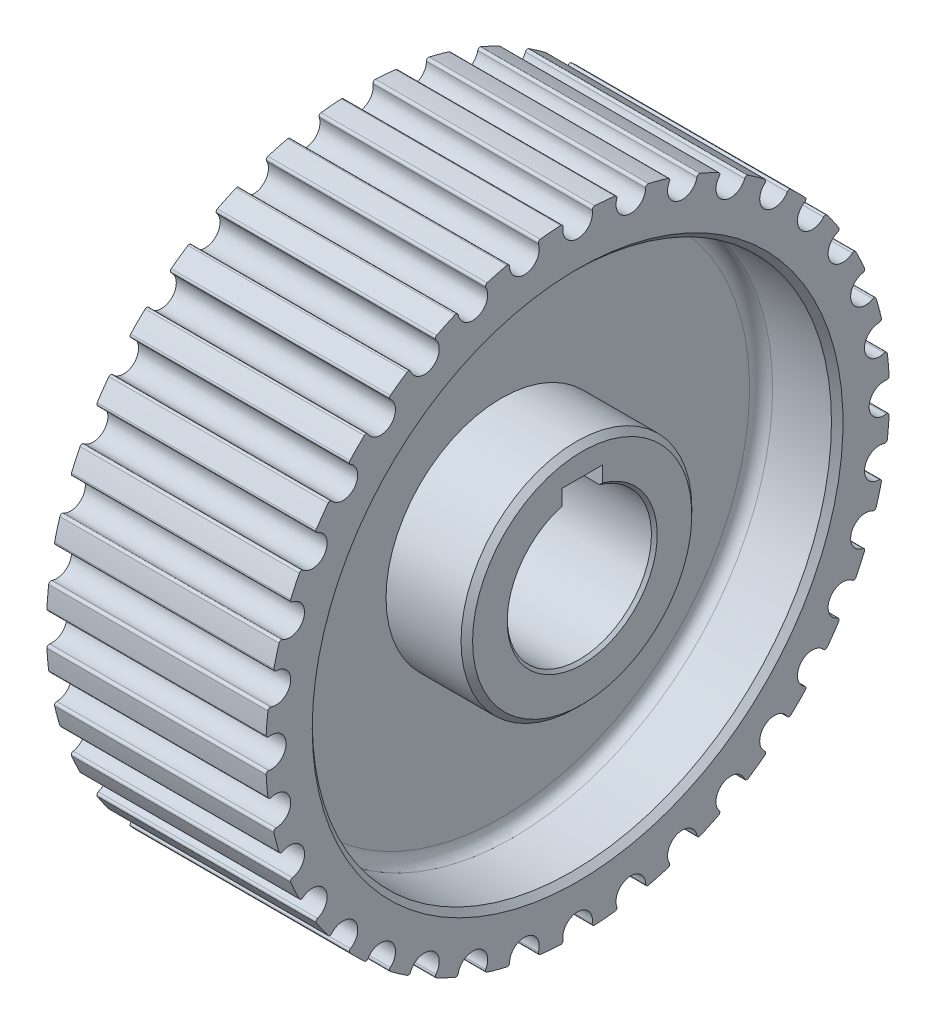
SolidWorks part; units mm, degrees
ref_plane "前视基准面" through (0, 0, 0) normal (0, 0, 1) x (1, 0, 0)
ref_plane "上视基准面" through (0, 0, 0) normal (0, 1, 0) x (1, 0, 0)
ref_plane "右视基准面" through (0, 0, 0) normal (1, 0, 0) x (0, 0, -1)
sketch "草图1" plane through (0, 0, 0) normal (0, 0, 1) x (1, 0, 0)
  line L0 (-38.4722, 0) -> (35.1779, 0) construction
  line L1 (-20.3293, 12.5) -> (17.6707, 12.5)
  line L2 (17.6707, 12.5) -> (17.6707, 20)
  line L3 (17.6707, 20) -> (3.6707, 20)
  line L4 (3.6707, 20) -> (3.6707, 45)
  line L5 (16.8769, 45) -> (3.6707, 45)
  line L6 (16.8769, 45) -> (16.8769, 54.07)
  line L7 (16.8769, 54.07) -> (-21.1231, 54.07)
  line L8 (-21.1231, 54.07) -> (-21.1231, 45)
  line L9 (-21.1231, 45) -> (-6.3293, 45)
  line L10 (-6.3293, 45) -> (-6.3293, 20)
  line L11 (-6.3293, 20) -> (-20.3293, 20)
  line L12 (-20.3293, 20) -> (-20.3293, 12.5)
  dimension "D1" = 38
  dimension "D2" = 7.5
  dimension "D3" = 14
  dimension "D4" = 14
  dimension "D5" = 7.5
  dimension "D6" = 25
  dimension "D7" = 9.07
  dimension "D8" = 12.5
revolve "旋转1" add sketch "草图1" angle 360 about L0
chamfer "倒角1" distance 1 angle 45 2 edges at (-21.1231, 0, 45) (16.8769, 0, 45)
fillet "圆角1" radius 2 2 edges at (-6.3293, 0, 45) (3.6707, 0, 45)
chamfer "倒角2" distance 1 angle 45 2 edges at (17.6707, 0, 20) (-20.3293, 0, 20)
chamfer "倒角3" distance 0.5 angle 45 2 edges at (-20.3293, 0, 12.5) (17.6707, 0, 12.5)
sketch "草图2" plane through (17.6707, 0, 0) normal (1, 0, 0) x (0, 0, -1)
  line L0 (0, -3.5835) -> (0, 27.7901) construction
  line L2 (-3.5, 12) -> (-3.5, 15.2)
  line L3 (-3.5, 15.2) -> (3.5, 15.2)
  line L4 (3.5, 12) -> (3.5, 15.2)
  arc A0 (3.5, 12) -> (-3.5, 12) centre (0, 0) ccw
  dimension "D1" = 25
  dimension "D2" = 3.2
  dimension "D3" = 7
  dimension "D4" = 3.5
extrude "切除-拉伸1" cut sketch "草图2" against normal through all
sketch "草图5" plane through (-21.1231, 0, 0) normal (-1, 0, 0) x (0, 0, 1)
  line L0 (0, 0) -> (0, 63.0632) construction
  arc A0 (-2.5348, 53.524) -> (2.5348, 53.524) centre (0, 53.1) ccw
  circle A1 centre (0, 0) radius 54.07 construction
  arc A2 (2.9511, 53.9894) -> (-2.9511, 53.9894) centre (0, 0) ccw
  arc A3 (-2.5348, 53.524) -> (-2.9511, 53.9894) centre (-2.9293, 53.59) ccw
  arc A4 (2.5348, 53.524) -> (2.9511, 53.9894) centre (2.9293, 53.59) cw
  point P8 (0, 50.53)
  point P9 (0, 54.07)
  point P12 (-2.5348, 53.524)
  dimension "D1" = 5.14
  dimension "D3" = 0.8
  dimension "D2" = 3.54
extrude "切除-拉伸2" cut sketch "草图5" against normal through all and the other way through all
pattern_circular "阵列(圆周)2" count 36 over 360 about axis through (0, 0, 0) along (1, 0, 0) of "切除-拉伸2"
sketch "草图6" plane through (-21.1231, 0, 0) normal (-1, 0, 0) x (0, 0, 1)
  arc A144 (-12.2815, 52.6567) -> (-15.6923, 51.7428) centre (0, 0) ccw
  arc A145 (-15.6923, 51.7428) -> (-15.9244, 51.1631) centre (-15.5762, 51.36) ccw
  arc A146 (-20.6882, 49.4292) -> (-15.9244, 51.1631) centre (-18.1613, 49.8977) ccw
  arc A147 (-20.6882, 49.4292) -> (-21.2386, 49.7241) centre (-21.0815, 49.3562) ccw
  arc A148 (-21.2386, 49.7241) -> (-24.4389, 48.2318) centre (0, 0) ccw
  arc A149 (-24.4389, 48.2318) -> (-24.5668, 47.6205) centre (-24.2582, 47.875) ccw
  arc A150 (-28.9572, 45.0858) -> (-24.5668, 47.6205) centre (-26.55, 45.9859) ccw
  arc A151 (-28.9572, 45.0858) -> (-29.5505, 45.2806) centre (-29.3318, 44.9457) ccw
  arc A152 (-29.5505, 45.2806) -> (-32.443, 43.2552) centre (0, 0) ccw
  arc A153 (-32.443, 43.2552) -> (-32.4628, 42.6311) centre (-32.203, 42.9352) ccw
  arc A154 (-36.3463, 39.3724) -> (-32.4628, 42.6311) centre (-34.132, 40.677) ccw
  arc A155 (-36.3463, 39.3724) -> (-36.9644, 39.4613) centre (-36.691, 39.1694) ccw
  arc A156 (-36.9644, 39.4613) -> (-39.4613, 36.9644) centre (0, 0) ccw
  arc A157 (-39.4613, 36.9644) -> (-39.3724, 36.3463) centre (-39.1694, 36.691) ccw
  arc A158 (-42.6311, 32.4628) -> (-39.3724, 36.3463) centre (-40.677, 34.132) ccw
  arc A159 (-42.6311, 32.4628) -> (-43.2552, 32.443) centre (-42.9352, 32.203) ccw
  arc A160 (-43.2552, 32.443) -> (-45.2806, 29.5505) centre (0, 0) ccw
  arc A161 (-45.2806, 29.5505) -> (-45.0858, 28.9572) centre (-44.9457, 29.3318) ccw
  arc A162 (-47.6205, 24.5668) -> (-45.0858, 28.9572) centre (-45.9859, 26.55) ccw
  arc A163 (-47.6205, 24.5668) -> (-48.2318, 24.4389) centre (-47.875, 24.2582) ccw
  arc A164 (-48.2318, 24.4389) -> (-49.7241, 21.2386) centre (0, 0) ccw
  arc A165 (-49.7241, 21.2386) -> (-49.4292, 20.6882) centre (-49.3562, 21.0815) ccw
  arc A166 (-51.1631, 15.9244) -> (-49.4292, 20.6882) centre (-49.8977, 18.1613) ccw
  arc A167 (-51.1631, 15.9244) -> (-51.7428, 15.6923) centre (-51.36, 15.5762) ccw
  arc A168 (-51.7428, 15.6923) -> (-52.6567, 12.2815) centre (0, 0) ccw
  arc A169 (-52.6567, 12.2815) -> (-52.2707, 11.7906) centre (-52.2672, 12.1906) ccw
  arc A170 (-53.151, 6.7981) -> (-52.2707, 11.7906) centre (-52.2933, 9.2207) ccw
  arc A171 (-53.151, 6.7981) -> (-53.6816, 6.4689) centre (-53.2845, 6.421) ccw
  arc A172 (-53.6816, 6.4689) -> (-53.9894, 2.9511) centre (0, 0) ccw
  arc A173 (-53.9894, 2.9511) -> (-53.524, 2.5348) centre (-53.59, 2.9293) ccw
  arc A174 (-53.524, -2.5348) -> (-53.524, 2.5348) centre (-53.1, 0) ccw
  arc A175 (-53.524, -2.5348) -> (-53.9894, -2.9511) centre (-53.59, -2.9293) ccw
  arc A176 (-53.9894, -2.9511) -> (-53.6816, -6.4689) centre (0, 0) ccw
  arc A177 (-53.6816, -6.4689) -> (-53.151, -6.7981) centre (-53.2845, -6.421) ccw
  arc A178 (-52.2707, -11.7906) -> (-53.151, -6.7981) centre (-52.2933, -9.2207) ccw
  arc A179 (-52.2707, -11.7906) -> (-52.6567, -12.2815) centre (-52.2672, -12.1906) ccw
  arc A180 (-52.6567, -12.2815) -> (-51.7428, -15.6923) centre (0, 0) ccw
  arc A181 (-51.7428, -15.6923) -> (-51.1631, -15.9244) centre (-51.36, -15.5762) ccw
  arc A182 (-49.4292, -20.6882) -> (-51.1631, -15.9244) centre (-49.8977, -18.1613) ccw
  arc A183 (-49.4292, -20.6882) -> (-49.7241, -21.2386) centre (-49.3562, -21.0815) ccw
  arc A184 (-49.7241, -21.2386) -> (-48.2318, -24.4389) centre (0, 0) ccw
  arc A185 (-48.2318, -24.4389) -> (-47.6205, -24.5668) centre (-47.875, -24.2582) ccw
  arc A186 (-45.0858, -28.9572) -> (-47.6205, -24.5668) centre (-45.9859, -26.55) ccw
  arc A187 (-45.0858, -28.9572) -> (-45.2806, -29.5505) centre (-44.9457, -29.3318) ccw
  arc A188 (-45.2806, -29.5505) -> (-43.2552, -32.443) centre (0, 0) ccw
  arc A189 (-43.2552, -32.443) -> (-42.6311, -32.4628) centre (-42.9352, -32.203) ccw
  arc A190 (-39.3724, -36.3463) -> (-42.6311, -32.4628) centre (-40.677, -34.132) ccw
  arc A191 (-39.3724, -36.3463) -> (-39.4613, -36.9644) centre (-39.1694, -36.691) ccw
  arc A192 (-39.4613, -36.9644) -> (-36.9644, -39.4613) centre (0, 0) ccw
  arc A193 (-36.9644, -39.4613) -> (-36.3463, -39.3724) centre (-36.691, -39.1694) ccw
  arc A194 (-32.4628, -42.6311) -> (-36.3463, -39.3724) centre (-34.132, -40.677) ccw
  arc A195 (-32.4628, -42.6311) -> (-32.443, -43.2552) centre (-32.203, -42.9352) ccw
  arc A196 (-32.443, -43.2552) -> (-29.5505, -45.2806) centre (0, 0) ccw
  arc A197 (-29.5505, -45.2806) -> (-28.9572, -45.0858) centre (-29.3318, -44.9457) ccw
  arc A198 (-24.5668, -47.6205) -> (-28.9572, -45.0858) centre (-26.55, -45.9859) ccw
  arc A199 (-24.5668, -47.6205) -> (-24.4389, -48.2318) centre (-24.2582, -47.875) ccw
  arc A200 (-24.4389, -48.2318) -> (-21.2386, -49.7241) centre (0, 0) ccw
  arc A201 (-21.2386, -49.7241) -> (-20.6882, -49.4292) centre (-21.0815, -49.3562) ccw
  arc A202 (-15.9244, -51.1631) -> (-20.6882, -49.4292) centre (-18.1613, -49.8977) ccw
  arc A203 (-15.9244, -51.1631) -> (-15.6923, -51.7428) centre (-15.5762, -51.36) ccw
  arc A204 (-15.6923, -51.7428) -> (-12.2815, -52.6567) centre (0, 0) ccw
  arc A205 (-12.2815, -52.6567) -> (-11.7906, -52.2707) centre (-12.1906, -52.2672) ccw
  arc A206 (-6.7981, -53.151) -> (-11.7906, -52.2707) centre (-9.2207, -52.2933) ccw
  arc A207 (-6.7981, -53.151) -> (-6.4689, -53.6816) centre (-6.421, -53.2845) ccw
  arc A208 (-6.4689, -53.6816) -> (-2.9511, -53.9894) centre (0, 0) ccw
  arc A209 (-2.9511, -53.9894) -> (-2.5348, -53.524) centre (-2.9293, -53.59) ccw
  arc A210 (2.5348, -53.524) -> (-2.5348, -53.524) centre (0, -53.1) ccw
  arc A211 (2.5348, -53.524) -> (2.9511, -53.9894) centre (2.9293, -53.59) ccw
  arc A212 (2.9511, -53.9894) -> (6.4689, -53.6816) centre (0, 0) ccw
  arc A213 (6.4689, -53.6816) -> (6.7981, -53.151) centre (6.421, -53.2845) ccw
  arc A214 (11.7906, -52.2707) -> (6.7981, -53.151) centre (9.2207, -52.2933) ccw
  arc A215 (11.7906, -52.2707) -> (12.2815, -52.6567) centre (12.1906, -52.2672) ccw
  arc A216 (12.2815, -52.6567) -> (15.6923, -51.7428) centre (0, 0) ccw
  arc A217 (15.6923, -51.7428) -> (15.9244, -51.1631) centre (15.5762, -51.36) ccw
  arc A218 (20.6882, -49.4292) -> (15.9244, -51.1631) centre (18.1613, -49.8977) ccw
  arc A219 (20.6882, -49.4292) -> (21.2386, -49.7241) centre (21.0815, -49.3562) ccw
  arc A220 (21.2386, -49.7241) -> (24.4389, -48.2318) centre (0, 0) ccw
  arc A221 (24.4389, -48.2318) -> (24.5668, -47.6205) centre (24.2582, -47.875) ccw
  arc A222 (28.9572, -45.0858) -> (24.5668, -47.6205) centre (26.55, -45.9859) ccw
  arc A223 (28.9572, -45.0858) -> (29.5505, -45.2806) centre (29.3318, -44.9457) ccw
  arc A224 (29.5505, -45.2806) -> (32.443, -43.2552) centre (0, 0) ccw
  arc A225 (32.443, -43.2552) -> (32.4628, -42.6311) centre (32.203, -42.9352) ccw
  arc A226 (36.3463, -39.3724) -> (32.4628, -42.6311) centre (34.132, -40.677) ccw
  arc A227 (36.3463, -39.3724) -> (36.9644, -39.4613) centre (36.691, -39.1694) ccw
  arc A228 (36.9644, -39.4613) -> (39.4613, -36.9644) centre (0, 0) ccw
  arc A229 (39.4613, -36.9644) -> (39.3724, -36.3463) centre (39.1694, -36.691) ccw
  arc A230 (42.6311, -32.4628) -> (39.3724, -36.3463) centre (40.677, -34.132) ccw
  arc A231 (42.6311, -32.4628) -> (43.2552, -32.443) centre (42.9352, -32.203) ccw
  arc A232 (43.2552, -32.443) -> (45.2806, -29.5505) centre (0, 0) ccw
  arc A233 (45.2806, -29.5505) -> (45.0858, -28.9572) centre (44.9457, -29.3318) ccw
  arc A234 (47.6205, -24.5668) -> (45.0858, -28.9572) centre (45.9859, -26.55) ccw
  arc A235 (47.6205, -24.5668) -> (48.2318, -24.4389) centre (47.875, -24.2582) ccw
  arc A236 (48.2318, -24.4389) -> (49.7241, -21.2386) centre (0, 0) ccw
  arc A237 (49.7241, -21.2386) -> (49.4292, -20.6882) centre (49.3562, -21.0815) ccw
  arc A238 (51.1631, -15.9244) -> (49.4292, -20.6882) centre (49.8977, -18.1613) ccw
  arc A239 (51.1631, -15.9244) -> (51.7428, -15.6923) centre (51.36, -15.5762) ccw
  arc A240 (51.7428, -15.6923) -> (52.6567, -12.2815) centre (0, 0) ccw
  arc A241 (52.6567, -12.2815) -> (52.2707, -11.7906) centre (52.2672, -12.1906) ccw
  arc A242 (53.151, -6.7981) -> (52.2707, -11.7906) centre (52.2933, -9.2207) ccw
  arc A243 (53.151, -6.7981) -> (53.6816, -6.4689) centre (53.2845, -6.421) ccw
  arc A244 (53.6816, -6.4689) -> (53.9894, -2.9511) centre (0, 0) ccw
  arc A245 (53.9894, -2.9511) -> (53.524, -2.5348) centre (53.59, -2.9293) ccw
  arc A246 (53.524, 2.5348) -> (53.524, -2.5348) centre (53.1, 0) ccw
  arc A247 (53.524, 2.5348) -> (53.9894, 2.9511) centre (53.59, 2.9293) ccw
  arc A248 (53.9894, 2.9511) -> (53.6816, 6.4689) centre (0, 0) ccw
  arc A249 (53.6816, 6.4689) -> (53.151, 6.7981) centre (53.2845, 6.421) ccw
  arc A250 (52.2707, 11.7906) -> (53.151, 6.7981) centre (52.2933, 9.2207) ccw
  arc A251 (52.2707, 11.7906) -> (52.6567, 12.2815) centre (52.2672, 12.1906) ccw
  arc A252 (52.6567, 12.2815) -> (51.7428, 15.6923) centre (0, 0) ccw
  arc A253 (51.7428, 15.6923) -> (51.1631, 15.9244) centre (51.36, 15.5762) ccw
  arc A254 (49.4292, 20.6882) -> (51.1631, 15.9244) centre (49.8977, 18.1613) ccw
  arc A255 (49.4292, 20.6882) -> (49.7241, 21.2386) centre (49.3562, 21.0815) ccw
  arc A256 (49.7241, 21.2386) -> (48.2318, 24.4389) centre (0, 0) ccw
  arc A257 (48.2318, 24.4389) -> (47.6205, 24.5668) centre (47.875, 24.2582) ccw
  arc A258 (45.0858, 28.9572) -> (47.6205, 24.5668) centre (45.9859, 26.55) ccw
  arc A259 (45.0858, 28.9572) -> (45.2806, 29.5505) centre (44.9457, 29.3318) ccw
  arc A260 (45.2806, 29.5505) -> (43.2552, 32.443) centre (0, 0) ccw
  arc A261 (43.2552, 32.443) -> (42.6311, 32.4628) centre (42.9352, 32.203) ccw
  arc A262 (39.3724, 36.3463) -> (42.6311, 32.4628) centre (40.677, 34.132) ccw
  arc A263 (39.3724, 36.3463) -> (39.4613, 36.9644) centre (39.1694, 36.691) ccw
  arc A264 (39.4613, 36.9644) -> (36.9644, 39.4613) centre (0, 0) ccw
  arc A265 (36.9644, 39.4613) -> (36.3463, 39.3724) centre (36.691, 39.1694) ccw
  arc A266 (32.4628, 42.6311) -> (36.3463, 39.3724) centre (34.132, 40.677) ccw
  arc A267 (32.4628, 42.6311) -> (32.443, 43.2552) centre (32.203, 42.9352) ccw
  arc A268 (32.443, 43.2552) -> (29.5505, 45.2806) centre (0, 0) ccw
  arc A269 (29.5505, 45.2806) -> (28.9572, 45.0858) centre (29.3318, 44.9457) ccw
  arc A270 (24.5668, 47.6205) -> (28.9572, 45.0858) centre (26.55, 45.9859) ccw
  arc A271 (24.5668, 47.6205) -> (24.4389, 48.2318) centre (24.2582, 47.875) ccw
  arc A272 (24.4389, 48.2318) -> (21.2386, 49.7241) centre (0, 0) ccw
  arc A273 (21.2386, 49.7241) -> (20.6882, 49.4292) centre (21.0815, 49.3562) ccw
  arc A274 (15.9244, 51.1631) -> (20.6882, 49.4292) centre (18.1613, 49.8977) ccw
  arc A275 (15.9244, 51.1631) -> (15.6923, 51.7428) centre (15.5762, 51.36) ccw
  arc A276 (15.6923, 51.7428) -> (12.2815, 52.6567) centre (0, 0) ccw
  arc A277 (12.2815, 52.6567) -> (11.7906, 52.2707) centre (12.1906, 52.2672) ccw
  arc A278 (6.7981, 53.151) -> (11.7906, 52.2707) centre (9.2207, 52.2933) ccw
  arc A279 (6.7981, 53.151) -> (6.4689, 53.6816) centre (6.421, 53.2845) ccw
  arc A280 (6.4689, 53.6816) -> (2.9511, 53.9894) centre (0, 0) ccw
  arc A281 (2.9511, 53.9894) -> (2.5348, 53.524) centre (2.9293, 53.59) ccw
  arc A282 (-2.5348, 53.524) -> (2.5348, 53.524) centre (0, 53.1) ccw
  arc A283 (-2.5348, 53.524) -> (-2.9511, 53.9894) centre (-2.9293, 53.59) ccw
  arc A284 (-2.9511, 53.9894) -> (-6.4689, 53.6816) centre (0, 0) ccw
  arc A285 (-6.4689, 53.6816) -> (-6.7981, 53.151) centre (-6.421, 53.2845) ccw
  arc A286 (-11.7906, 52.2707) -> (-6.7981, 53.151) centre (-9.2207, 52.2933) ccw
  arc A287 (-11.7906, 52.2707) -> (-12.2815, 52.6567) centre (-12.1906, 52.2672) ccw
  arc A288 (-12.2815, 52.6567) -> (-15.6923, 51.7428) centre (0, 0) ccw
  arc A289 (-15.6923, 51.7428) -> (-15.9244, 51.1631) centre (-15.5762, 51.36) ccw
  arc A290 (-20.6882, 49.4292) -> (-15.9244, 51.1631) centre (-18.1613, 49.8977) ccw
  arc A291 (-20.6882, 49.4292) -> (-21.2386, 49.7241) centre (-21.0815, 49.3562) ccw
  arc A292 (-21.2386, 49.7241) -> (-24.4389, 48.2318) centre (0, 0) ccw
  arc A293 (-24.4389, 48.2318) -> (-24.5668, 47.6205) centre (-24.2582, 47.875) ccw
  arc A294 (-28.9572, 45.0858) -> (-24.5668, 47.6205) centre (-26.55, 45.9859) ccw
  arc A295 (-28.9572, 45.0858) -> (-29.5505, 45.2806) centre (-29.3318, 44.9457) ccw
  arc A296 (-29.5505, 45.2806) -> (-32.443, 43.2552) centre (0, 0) ccw
  arc A297 (-32.443, 43.2552) -> (-32.4628, 42.6311) centre (-32.203, 42.9352) ccw
  arc A298 (-36.3463, 39.3724) -> (-32.4628, 42.6311) centre (-34.132, 40.677) ccw
  arc A299 (-36.3463, 39.3724) -> (-36.9644, 39.4613) centre (-36.691, 39.1694) ccw
  arc A300 (-36.9644, 39.4613) -> (-39.4613, 36.9644) centre (0, 0) ccw
  arc A301 (-39.4613, 36.9644) -> (-39.3724, 36.3463) centre (-39.1694, 36.691) ccw
  arc A302 (-42.6311, 32.4628) -> (-39.3724, 36.3463) centre (-40.677, 34.132) ccw
  arc A303 (-42.6311, 32.4628) -> (-43.2552, 32.443) centre (-42.9352, 32.203) ccw
  arc A304 (-43.2552, 32.443) -> (-45.2806, 29.5505) centre (0, 0) ccw
  arc A305 (-45.2806, 29.5505) -> (-45.0858, 28.9572) centre (-44.9457, 29.3318) ccw
  arc A306 (-47.6205, 24.5668) -> (-45.0858, 28.9572) centre (-45.9859, 26.55) ccw
  arc A307 (-47.6205, 24.5668) -> (-48.2318, 24.4389) centre (-47.875, 24.2582) ccw
  arc A308 (-48.2318, 24.4389) -> (-49.7241, 21.2386) centre (0, 0) ccw
  arc A309 (-49.7241, 21.2386) -> (-49.4292, 20.6882) centre (-49.3562, 21.0815) ccw
  arc A310 (-51.1631, 15.9244) -> (-49.4292, 20.6882) centre (-49.8977, 18.1613) ccw
  arc A311 (-51.1631, 15.9244) -> (-51.7428, 15.6923) centre (-51.36, 15.5762) ccw
  arc A312 (-51.7428, 15.6923) -> (-52.6567, 12.2815) centre (0, 0) ccw
  arc A313 (-52.6567, 12.2815) -> (-52.2707, 11.7906) centre (-52.2672, 12.1906) ccw
  arc A314 (-53.151, 6.7981) -> (-52.2707, 11.7906) centre (-52.2933, 9.2207) ccw
  arc A315 (-53.151, 6.7981) -> (-53.6816, 6.4689) centre (-53.2845, 6.421) ccw
  arc A316 (-53.6816, 6.4689) -> (-53.9894, 2.9511) centre (0, 0) ccw
  arc A317 (-53.9894, 2.9511) -> (-53.524, 2.5348) centre (-53.59, 2.9293) ccw
  arc A318 (-53.524, -2.5348) -> (-53.524, 2.5348) centre (-53.1, 0) ccw
  arc A319 (-53.524, -2.5348) -> (-53.9894, -2.9511) centre (-53.59, -2.9293) ccw
  arc A320 (-53.9894, -2.9511) -> (-53.6816, -6.4689) centre (0, 0) ccw
  arc A321 (-53.6816, -6.4689) -> (-53.151, -6.7981) centre (-53.2845, -6.421) ccw
  arc A322 (-52.2707, -11.7906) -> (-53.151, -6.7981) centre (-52.2933, -9.2207) ccw
  arc A323 (-52.2707, -11.7906) -> (-52.6567, -12.2815) centre (-52.2672, -12.1906) ccw
  arc A324 (-52.6567, -12.2815) -> (-51.7428, -15.6923) centre (0, 0) ccw
  arc A325 (-51.7428, -15.6923) -> (-51.1631, -15.9244) centre (-51.36, -15.5762) ccw
  arc A326 (-49.4292, -20.6882) -> (-51.1631, -15.9244) centre (-49.8977, -18.1613) ccw
  arc A327 (-49.4292, -20.6882) -> (-49.7241, -21.2386) centre (-49.3562, -21.0815) ccw
  arc A328 (-49.7241, -21.2386) -> (-48.2318, -24.4389) centre (0, 0) ccw
  arc A329 (-48.2318, -24.4389) -> (-47.6205, -24.5668) centre (-47.875, -24.2582) ccw
  arc A330 (-45.0858, -28.9572) -> (-47.6205, -24.5668) centre (-45.9859, -26.55) ccw
  arc A331 (-45.0858, -28.9572) -> (-45.2806, -29.5505) centre (-44.9457, -29.3318) ccw
  arc A332 (-45.2806, -29.5505) -> (-43.2552, -32.443) centre (0, 0) ccw
  arc A333 (-43.2552, -32.443) -> (-42.6311, -32.4628) centre (-42.9352, -32.203) ccw
  arc A334 (-39.3724, -36.3463) -> (-42.6311, -32.4628) centre (-40.677, -34.132) ccw
  arc A335 (-39.3724, -36.3463) -> (-39.4613, -36.9644) centre (-39.1694, -36.691) ccw
  arc A336 (-39.4613, -36.9644) -> (-36.9644, -39.4613) centre (0, 0) ccw
  arc A337 (-36.9644, -39.4613) -> (-36.3463, -39.3724) centre (-36.691, -39.1694) ccw
  arc A338 (-32.4628, -42.6311) -> (-36.3463, -39.3724) centre (-34.132, -40.677) ccw
  arc A339 (-32.4628, -42.6311) -> (-32.443, -43.2552) centre (-32.203, -42.9352) ccw
  arc A340 (-32.443, -43.2552) -> (-29.5505, -45.2806) centre (0, 0) ccw
  arc A341 (-29.5505, -45.2806) -> (-28.9572, -45.0858) centre (-29.3318, -44.9457) ccw
  arc A342 (-24.5668, -47.6205) -> (-28.9572, -45.0858) centre (-26.55, -45.9859) ccw
  arc A343 (-24.5668, -47.6205) -> (-24.4389, -48.2318) centre (-24.2582, -47.875) ccw
  arc A344 (-24.4389, -48.2318) -> (-21.2386, -49.7241) centre (0, 0) ccw
  arc A345 (-21.2386, -49.7241) -> (-20.6882, -49.4292) centre (-21.0815, -49.3562) ccw
  arc A346 (-15.9244, -51.1631) -> (-20.6882, -49.4292) centre (-18.1613, -49.8977) ccw
  arc A347 (-15.9244, -51.1631) -> (-15.6923, -51.7428) centre (-15.5762, -51.36) ccw
  arc A348 (-15.6923, -51.7428) -> (-12.2815, -52.6567) centre (0, 0) ccw
  arc A349 (-12.2815, -52.6567) -> (-11.7906, -52.2707) centre (-12.1906, -52.2672) ccw
  arc A350 (-6.7981, -53.151) -> (-11.7906, -52.2707) centre (-9.2207, -52.2933) ccw
  arc A351 (-6.7981, -53.151) -> (-6.4689, -53.6816) centre (-6.421, -53.2845) ccw
  arc A352 (-6.4689, -53.6816) -> (-2.9511, -53.9894) centre (0, 0) ccw
  arc A353 (-2.9511, -53.9894) -> (-2.5348, -53.524) centre (-2.9293, -53.59) ccw
  arc A354 (2.5348, -53.524) -> (-2.5348, -53.524) centre (0, -53.1) ccw
  arc A355 (2.5348, -53.524) -> (2.9511, -53.9894) centre (2.9293, -53.59) ccw
  arc A356 (2.9511, -53.9894) -> (6.4689, -53.6816) centre (0, 0) ccw
  arc A357 (6.4689, -53.6816) -> (6.7981, -53.151) centre (6.421, -53.2845) ccw
  arc A358 (11.7906, -52.2707) -> (6.7981, -53.151) centre (9.2207, -52.2933) ccw
  arc A359 (11.7906, -52.2707) -> (12.2815, -52.6567) centre (12.1906, -52.2672) ccw
  arc A360 (12.2815, -52.6567) -> (15.6923, -51.7428) centre (0, 0) ccw
  arc A361 (15.6923, -51.7428) -> (15.9244, -51.1631) centre (15.5762, -51.36) ccw
  arc A362 (20.6882, -49.4292) -> (15.9244, -51.1631) centre (18.1613, -49.8977) ccw
  arc A363 (20.6882, -49.4292) -> (21.2386, -49.7241) centre (21.0815, -49.3562) ccw
  arc A364 (21.2386, -49.7241) -> (24.4389, -48.2318) centre (0, 0) ccw
  arc A365 (24.4389, -48.2318) -> (24.5668, -47.6205) centre (24.2582, -47.875) ccw
  arc A366 (28.9572, -45.0858) -> (24.5668, -47.6205) centre (26.55, -45.9859) ccw
  arc A367 (28.9572, -45.0858) -> (29.5505, -45.2806) centre (29.3318, -44.9457) ccw
  arc A368 (29.5505, -45.2806) -> (32.443, -43.2552) centre (0, 0) ccw
  arc A369 (32.443, -43.2552) -> (32.4628, -42.6311) centre (32.203, -42.9352) ccw
  arc A370 (36.3463, -39.3724) -> (32.4628, -42.6311) centre (34.132, -40.677) ccw
  arc A371 (36.3463, -39.3724) -> (36.9644, -39.4613) centre (36.691, -39.1694) ccw
  arc A372 (36.9644, -39.4613) -> (39.4613, -36.9644) centre (0, 0) ccw
  arc A373 (39.4613, -36.9644) -> (39.3724, -36.3463) centre (39.1694, -36.691) ccw
  arc A374 (42.6311, -32.4628) -> (39.3724, -36.3463) centre (40.677, -34.132) ccw
  arc A375 (42.6311, -32.4628) -> (43.2552, -32.443) centre (42.9352, -32.203) ccw
  arc A376 (43.2552, -32.443) -> (45.2806, -29.5505) centre (0, 0) ccw
  arc A377 (45.2806, -29.5505) -> (45.0858, -28.9572) centre (44.9457, -29.3318) ccw
  arc A378 (47.6205, -24.5668) -> (45.0858, -28.9572) centre (45.9859, -26.55) ccw
  arc A379 (47.6205, -24.5668) -> (48.2318, -24.4389) centre (47.875, -24.2582) ccw
  arc A380 (48.2318, -24.4389) -> (49.7241, -21.2386) centre (0, 0) ccw
  arc A381 (49.7241, -21.2386) -> (49.4292, -20.6882) centre (49.3562, -21.0815) ccw
  arc A382 (51.1631, -15.9244) -> (49.4292, -20.6882) centre (49.8977, -18.1613) ccw
  arc A383 (51.1631, -15.9244) -> (51.7428, -15.6923) centre (51.36, -15.5762) ccw
  arc A384 (51.7428, -15.6923) -> (52.6567, -12.2815) centre (0, 0) ccw
  arc A385 (52.6567, -12.2815) -> (52.2707, -11.7906) centre (52.2672, -12.1906) ccw
  arc A386 (53.151, -6.7981) -> (52.2707, -11.7906) centre (52.2933, -9.2207) ccw
  arc A387 (53.151, -6.7981) -> (53.6816, -6.4689) centre (53.2845, -6.421) ccw
  arc A388 (53.6816, -6.4689) -> (53.9894, -2.9511) centre (0, 0) ccw
  arc A389 (53.9894, -2.9511) -> (53.524, -2.5348) centre (53.59, -2.9293) ccw
  arc A390 (53.524, 2.5348) -> (53.524, -2.5348) centre (53.1, 0) ccw
  arc A391 (53.524, 2.5348) -> (53.9894, 2.9511) centre (53.59, 2.9293) ccw
  arc A392 (53.9894, 2.9511) -> (53.6816, 6.4689) centre (0, 0) ccw
  arc A393 (53.6816, 6.4689) -> (53.151, 6.7981) centre (53.2845, 6.421) ccw
  arc A394 (52.2707, 11.7906) -> (53.151, 6.7981) centre (52.2933, 9.2207) ccw
  arc A395 (52.2707, 11.7906) -> (52.6567, 12.2815) centre (52.2672, 12.1906) ccw
  arc A396 (52.6567, 12.2815) -> (51.7428, 15.6923) centre (0, 0) ccw
  arc A397 (51.7428, 15.6923) -> (51.1631, 15.9244) centre (51.36, 15.5762) ccw
  arc A398 (49.4292, 20.6882) -> (51.1631, 15.9244) centre (49.8977, 18.1613) ccw
  arc A399 (49.4292, 20.6882) -> (49.7241, 21.2386) centre (49.3562, 21.0815) ccw
  arc A400 (49.7241, 21.2386) -> (48.2318, 24.4389) centre (0, 0) ccw
  arc A401 (48.2318, 24.4389) -> (47.6205, 24.5668) centre (47.875, 24.2582) ccw
  arc A402 (45.0858, 28.9572) -> (47.6205, 24.5668) centre (45.9859, 26.55) ccw
  arc A403 (45.0858, 28.9572) -> (45.2806, 29.5505) centre (44.9457, 29.3318) ccw
  arc A404 (45.2806, 29.5505) -> (43.2552, 32.443) centre (0, 0) ccw
  arc A405 (43.2552, 32.443) -> (42.6311, 32.4628) centre (42.9352, 32.203) ccw
  arc A406 (39.3724, 36.3463) -> (42.6311, 32.4628) centre (40.677, 34.132) ccw
  arc A407 (39.3724, 36.3463) -> (39.4613, 36.9644) centre (39.1694, 36.691) ccw
  arc A408 (39.4613, 36.9644) -> (36.9644, 39.4613) centre (0, 0) ccw
  arc A409 (36.9644, 39.4613) -> (36.3463, 39.3724) centre (36.691, 39.1694) ccw
  arc A410 (32.4628, 42.6311) -> (36.3463, 39.3724) centre (34.132, 40.677) ccw
  arc A411 (32.4628, 42.6311) -> (32.443, 43.2552) centre (32.203, 42.9352) ccw
  arc A412 (32.443, 43.2552) -> (29.5505, 45.2806) centre (0, 0) ccw
  arc A413 (29.5505, 45.2806) -> (28.9572, 45.0858) centre (29.3318, 44.9457) ccw
  arc A414 (24.5668, 47.6205) -> (28.9572, 45.0858) centre (26.55, 45.9859) ccw
  arc A415 (24.5668, 47.6205) -> (24.4389, 48.2318) centre (24.2582, 47.875) ccw
  arc A416 (24.4389, 48.2318) -> (21.2386, 49.7241) centre (0, 0) ccw
  arc A417 (21.2386, 49.7241) -> (20.6882, 49.4292) centre (21.0815, 49.3562) ccw
  arc A418 (15.9244, 51.1631) -> (20.6882, 49.4292) centre (18.1613, 49.8977) ccw
  arc A419 (15.9244, 51.1631) -> (15.6923, 51.7428) centre (15.5762, 51.36) ccw
  arc A420 (15.6923, 51.7428) -> (12.2815, 52.6567) centre (0, 0) ccw
  arc A421 (12.2815, 52.6567) -> (11.7906, 52.2707) centre (12.1906, 52.2672) ccw
  arc A422 (6.7981, 53.151) -> (11.7906, 52.2707) centre (9.2207, 52.2933) ccw
  arc A423 (6.7981, 53.151) -> (6.4689, 53.6816) centre (6.421, 53.2845) ccw
  arc A424 (6.4689, 53.6816) -> (2.9511, 53.9894) centre (0, 0) ccw
  arc A425 (2.9511, 53.9894) -> (2.5348, 53.524) centre (2.9293, 53.59) ccw
  arc A426 (-2.5348, 53.524) -> (2.5348, 53.524) centre (0, 53.1) ccw
  arc A427 (-2.5348, 53.524) -> (-2.9511, 53.9894) centre (-2.9293, 53.59) ccw
  arc A428 (-2.9511, 53.9894) -> (-6.4689, 53.6816) centre (0, 0) ccw
  arc A429 (-6.4689, 53.6816) -> (-6.7981, 53.151) centre (-6.421, 53.2845) ccw
  arc A430 (-11.7906, 52.2707) -> (-6.7981, 53.151) centre (-9.2207, 52.2933) ccw
  arc A431 (-11.7906, 52.2707) -> (-12.2815, 52.6567) centre (-12.1906, 52.2672) ccw
  dimension "D1" = 0
